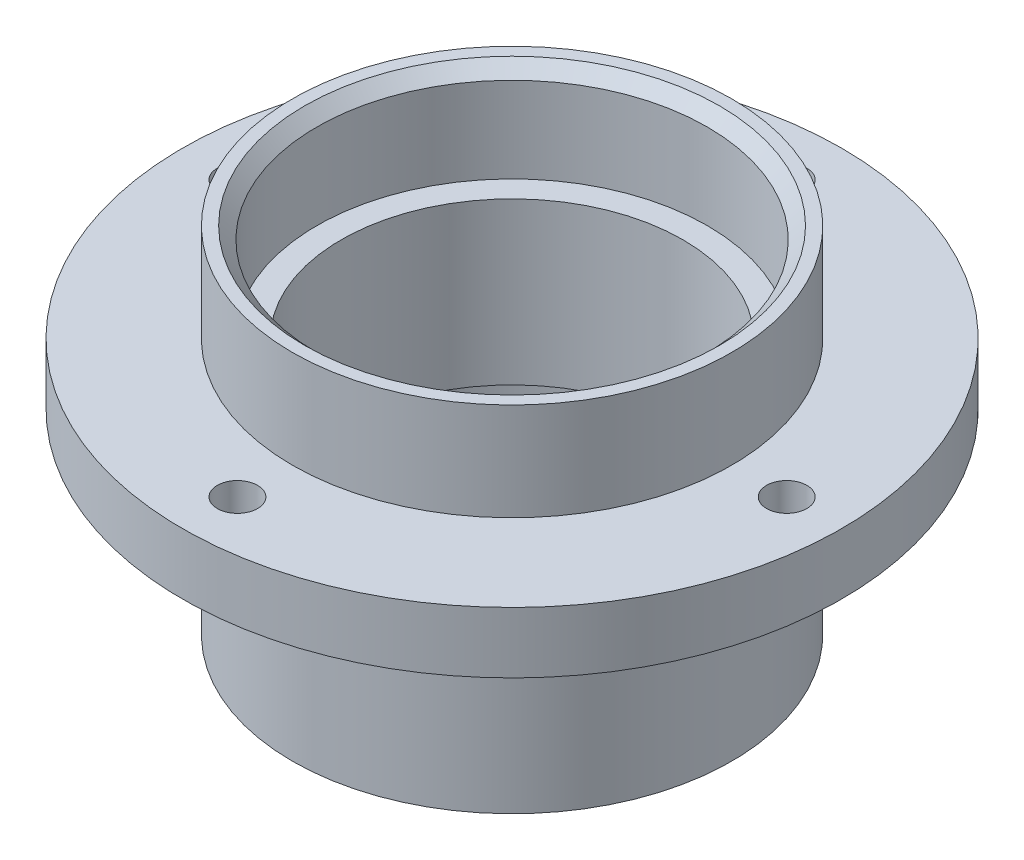
SolidWorks part; units mm, degrees
material "尼龙 101"
ref_plane "Front Plane" through (0, 0, 0) normal (0, 0, 1) x (1, 0, 0)
ref_plane "Top Plane" through (0, 0, 0) normal (0, 1, 0) x (1, 0, 0)
ref_plane "Right Plane" through (0, 0, 0) normal (1, 0, 0) x (0, 0, -1)
sketch "Sketch1" plane through (0, 0, 0) normal (0, 1, 0) x (1, 0, 0)
  circle A0 centre (0, 0) radius 18
  dimension "D1" = 36
extrude "Boss-Extrude1" add sketch "Sketch1" along normal blind 8
sketch "Sketch2" plane through (0, 0, 0) normal (0, -1, 0) x (1, 0, 0)
  circle A0 centre (0, 0) radius 16
  dimension "D1" = 32
extrude "Cut-Extrude1" cut sketch "Sketch2" against normal up to next
sketch "Sketch3" plane through (0, 0, 0) normal (0, -1, 0) x (1, 0, 0)
  circle A0 centre (0, 0) radius 27
  dimension "D1" = 54
extrude "Boss-Extrude2" add sketch "Sketch3" along normal blind 5
sketch "Sketch4" plane through (0, -5, 0) normal (0, -1, 0) x (1, 0, 0)
  circle A0 centre (0, 0) radius 18
  dimension "D1" = 36
extrude "Boss-Extrude3" add sketch "Sketch4" along normal blind 16
sketch "Sketch5" plane through (0, -21, 0) normal (0, -1, 0) x (1, 0, 0)
  circle A0 centre (0, 0) radius 16
  dimension "D1" = 32
extrude "Cut-Extrude2" cut sketch "Sketch5" against normal blind 7.8
sketch "Sketch6" plane through (0, 0, 0) normal (0, 1, 0) x (1, 0, 0)
  circle A0 centre (0, 0) radius 14
  dimension "D1" = 28
extrude "Cut-Extrude3" cut sketch "Sketch6" against normal through all
hole_wizard "M4 Tapped Hole1" positions "Sketch8" profile "Sketch7" tap size "M4" standard "GB"
sketch "Sketch8" plane through (0, 0, 0) normal (0, 1, 0) x (1, 0, 0)
  line L0 (0, 0) -> (34.4413, 0) construction
  line L2 (0, 0) -> (0, -34.4413) construction
  line L3 (0, 0) -> (-34.4413, 0) construction
  line L4 (0, 0) -> (0, 34.4413) construction
  circle A0 centre (0, 0) radius 22.5 construction
  point P0 (-22.5, 0)
  point P11 (0, 0)
  point P16 (0, 22.5)
  point P18 (22.5, 0)
  point P20 (0, -22.5)
  dimension "D1" = 45
  dimension "D2" = 4
cosmetic thread "Cosmetic Thread1" parameters "D1"=5, "D2"=4
cosmetic thread "Cosmetic Thread2" parameters "D1"=5, "D2"=4
cosmetic thread "Cosmetic Thread3" parameters "D1"=5, "D2"=4
cosmetic thread "Cosmetic Thread4" parameters "D1"=5, "D2"=4
sketch "Sketch7" plane through (-22.5, 0, 0) normal (1, 0, 0) x (0, 0, 1)
  line L0 (0, 0) -> (0, 12.4914)
  line L1 (0, 12.4914) -> (1.65, 11.5)
  line L2 (1.65, 11.5) -> (1.65, 0)
  line L5 (1.65, 0) -> (0, 0)
  line L10 (0, 12.4914) -> (-1.65, 11.5) construction
  line L11 (0, -6.35) -> (0, 107.95) construction
  dimension "螺纹孔钻头直径" = 3.3
  dimension "螺纹孔钻头深度" = 11.5
  dimension "导头角度" = 118
chamfer "Chamfer1" distance 1 angle 45 2 edges at (0, -21, -16) (0, 8, 16)
